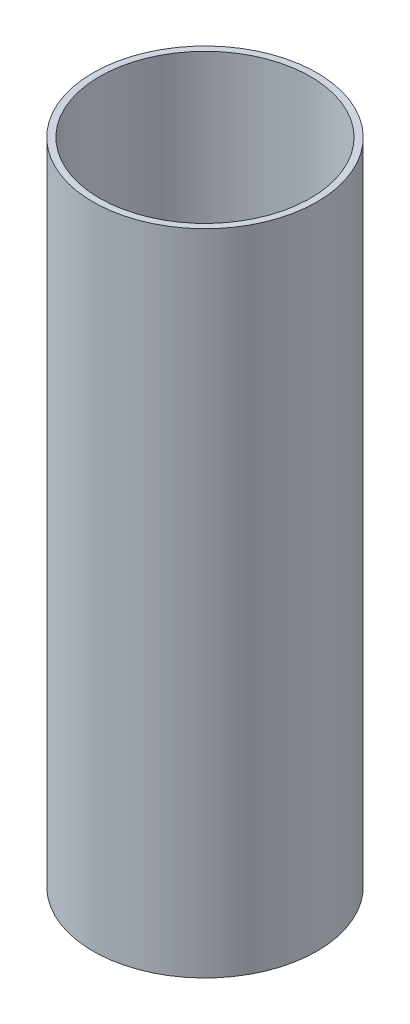
SolidWorks part; units mm, degrees
material "ABS"
ref_plane "Front Plane" through (0, 0, 0) normal (0, 0, 1) x (1, 0, 0)
ref_plane "Top Plane" through (0, 0, 0) normal (0, 1, 0) x (1, 0, 0)
ref_plane "Right Plane" through (0, 0, 0) normal (1, 0, 0) x (0, 0, -1)
sketch "Sketch1" plane through (0, 0, 0) normal (0, 1, 0) x (1, 0, 0)
  circle A0 centre (0, 0) radius 3.25
  dimension "D1" = 6.5
extrude "Extrude-Thin1" add sketch "Sketch1" along normal blind 20 thin
